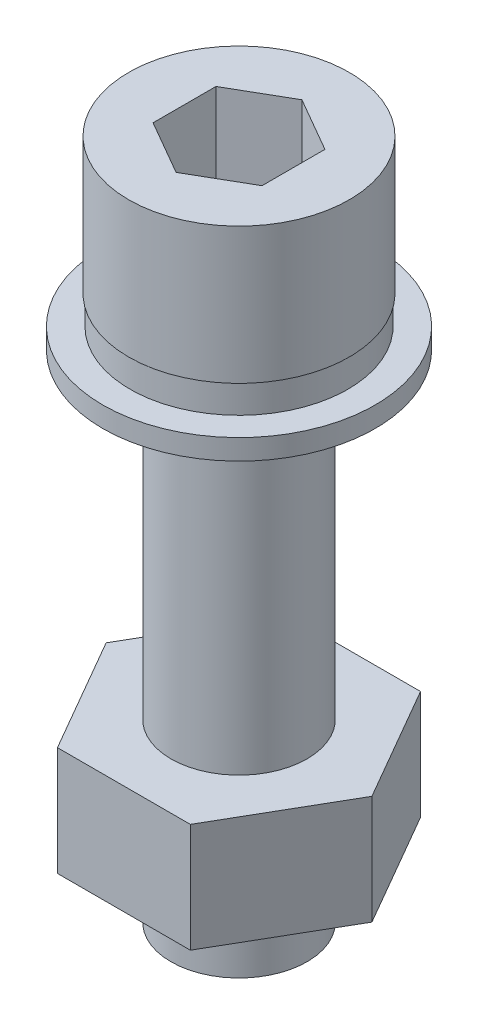
from build123d import *

# Parameters (mm, degrees)
CUT_EXTRUDE_1_DEPTH  = 6
SKETCH_3_R           = 8
SKETCH_3_R_2         = 5
BOSS_EXTRUDE_1_DEPTH = 2.1
SKETCH_4_R           = 10
SKETCH_4_R_2         = 5
BOSS_EXTRUDE_2_DEPTH = 1.5
BOSS_EXTRUDE_START   = 8
SKETCH_5_R           = 5
BOSS_EXTRUDE_3_DEPTH = 8


with BuildPart() as part:
    # Sketch 1 → Revolve 1 (revolve)
    with BuildSketch(Plane.XY, mode=Mode.PRIVATE) as revolve_1_sk:
        Polygon((0, 10), (-8.1, 10), (-8.1, 0), (-5, 0), (-5, -40), (0, -40), align=None)
    revolve(revolve_1_sk.sketch.rotate(Axis((0, 11.322033898, 0), (0, -1, 0)), 270), axis=Axis((0, 11.322033898, 0), (0, -1, 0)))

    # Sketch 2 → Cut-Extrude 1 (cut)
    with BuildSketch(Plane(origin=(0, 10, 0), x_dir=(1, 0, 0), z_dir=(0, 1, 0))):
        Polygon((0, 4.618802154), (-4, 2.309401077), (-4, -2.309401077), (0, -4.618802154), (4, -2.309401077), (4, 2.309401077), align=None)
    extrude(amount=-CUT_EXTRUDE_1_DEPTH, mode=Mode.SUBTRACT)

    # Sketch 5 → Boss-Extrude 3 (add)
    with BuildSketch(Plane(origin=(0, -27.1, 0), x_dir=(-1, 0, 0), z_dir=(0, -1, 0)).offset(BOSS_EXTRUDE_START)):
        Polygon((-9.757219549, 0), (-4.878609775, -8.45), (4.878609775, -8.45), (9.757219549, 0), (4.878609775, 8.45), (-4.878609775, 8.45), align=None)
        with Locations(Location((0, 0, 0), (0, 0, 90))):
            Circle(SKETCH_5_R, mode=Mode.SUBTRACT)
    extrude(amount=-BOSS_EXTRUDE_3_DEPTH)


with BuildPart() as body_2:
    # Sketch 3 → Boss-Extrude 1 (new body)
    with BuildSketch(Plane.XZ):
        with Locations(Location((0, 0, 0), (0, 0, 270))):
            Circle(SKETCH_3_R)
        with Locations(Location((0, 0, 0), (0, 0, 270))):
            Circle(SKETCH_3_R_2, mode=Mode.SUBTRACT)
    extrude(amount=BOSS_EXTRUDE_1_DEPTH)


with BuildPart() as body_3:
    # Sketch 4 → Boss-Extrude 2 (new body)
    with BuildSketch(Plane.XZ.offset(2.1)):
        with Locations(Location((0, 0, 0), (0, 0, 270))):
            Circle(SKETCH_4_R)
        with Locations(Location((0, 0, 0), (0, 0, 270))):
            Circle(SKETCH_4_R_2, mode=Mode.SUBTRACT)
    extrude(amount=BOSS_EXTRUDE_2_DEPTH)


solid = Compound([part.part, body_2.part, body_3.part])
